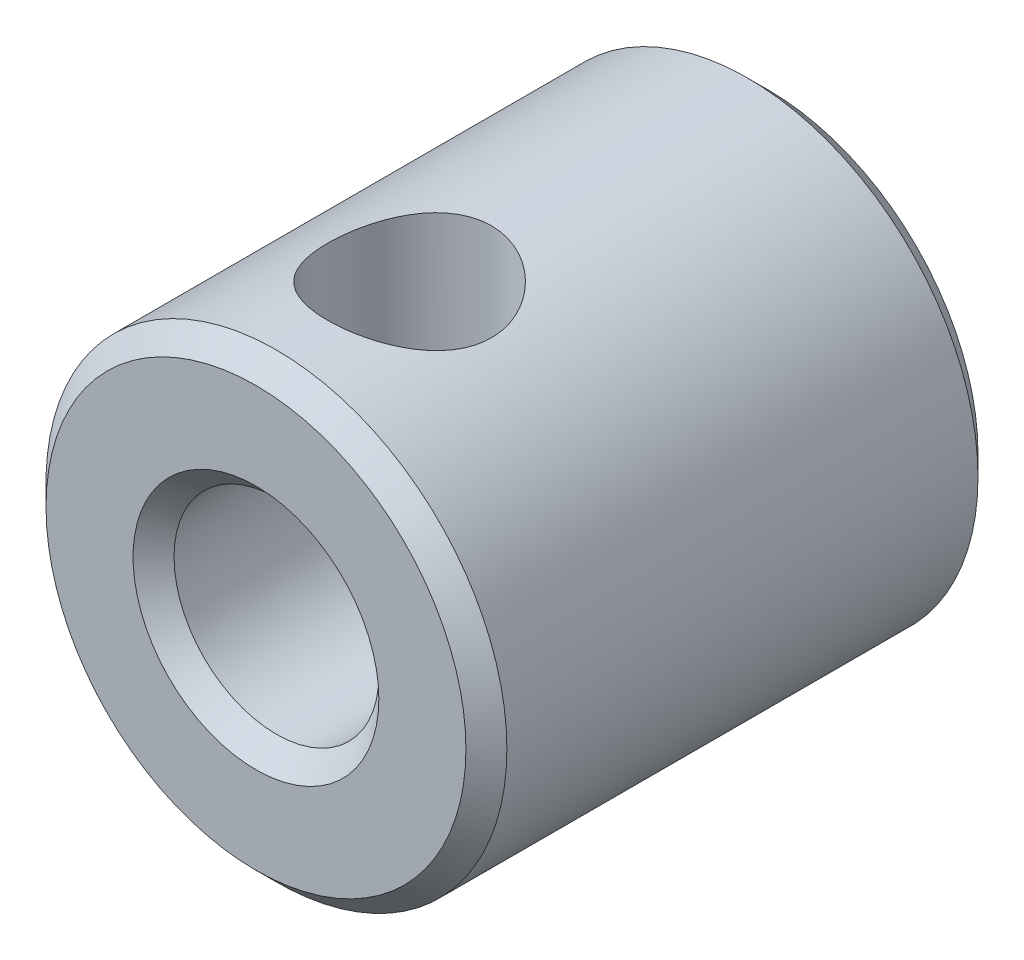
SolidWorks part; units mm, degrees
ref_plane "Front Plane" through (0, 0, 0) normal (0, 0, 1) x (1, 0, 0)
ref_plane "Top Plane" through (0, 0, 0) normal (0, 1, 0) x (1, 0, 0)
ref_plane "Right Plane" through (0, 0, 0) normal (1, 0, 0) x (0, 0, -1)
sketch "Sketch1" plane through (0, 0, 0) normal (0, 0, 1) x (1, 0, 0)
  circle A0 centre (0, 0) radius 2.25
  circle A1 centre (0, 0) radius 1
  dimension "D1" = 2
  dimension "D2" = 4.5
extrude "Boss-Extrude1" add sketch "Sketch1" along normal mid plane 5
chamfer "Chamfer1" distance 0.2 angle 45 4 edges at (2.25, 0, -2.5) (2.25, 0, 2.5) (1, 0, -2.5) (1, 0, 2.5)
hole_wizard "M2 Tapped Hole1" positions "Sketch3" profile "Sketch2" tap size "M2" standard "Gb"
sketch "Sketch3" plane through (0, 0, 0) normal (0, 1, 0) x (1, 0, 0)
  line L1 (-2.05, -2.5) -> (2.05, -2.5) construction
  point P0 (0, -1)
  dimension "D1" = 1.5
sketch "Sketch2" plane through (0, 0, 1) normal (1, 0, 0) x (0, 0, -1)
  line L0 (0, 0) -> (0, 2.25)
  line L1 (0, 2.25) -> (0.8, 2.25)
  line L2 (0.8, 2.25) -> (0.8, 0)
  line L5 (0.8, 0) -> (0, 0)
  line L11 (0, -6.35) -> (0, 107.95) construction
  dimension "通孔螺纹孔钻头直径" = 1.6
  dimension "通孔螺纹孔钻头深度" = 2.25
cosmetic thread "Hole Thread2" parameters "D2"=2
